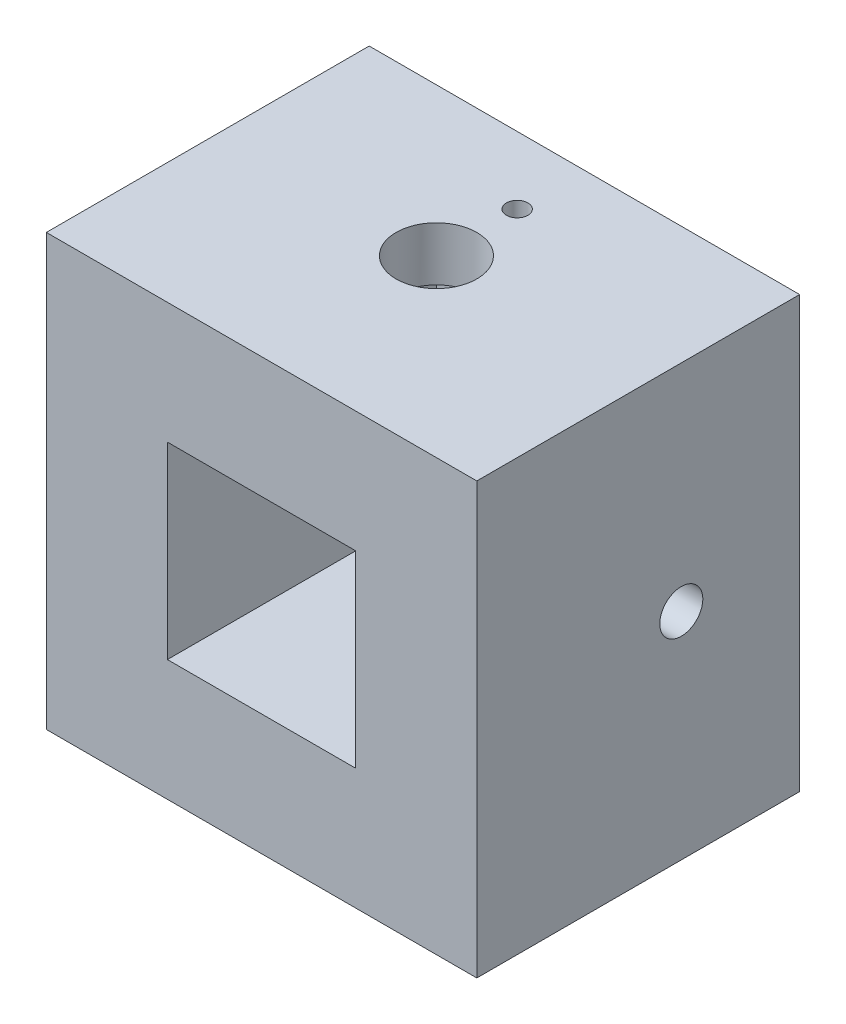
SolidWorks part; units mm, degrees
ref_plane "Front Plane" through (0, 0, 0) normal (0, 0, 1) x (1, 0, 0)
ref_plane "Top Plane" through (0, 0, 0) normal (0, 1, 0) x (1, 0, 0)
ref_plane "Right Plane" through (0, 0, 0) normal (1, 0, 0) x (0, 0, -1)
sketch "Sketch1" plane through (0, 0, 0) normal (0, 0, 1) x (1, 0, 0)
  line L1 (-51.5, -61.5) -> (-131.5, -61.5)
  line L2 (-51.5, -61.5) -> (-51.5, 18.5)
  line L3 (-51.5, 18.5) -> (-131.5, 18.5)
  line L4 (-131.5, -61.5) -> (-131.5, 18.5)
  line L5 (-51.5, -61.5) -> (-131.5, 18.5) construction
  line L6 (-51.5, 18.5) -> (-131.5, -61.5) construction
  point P0 (-91.5, -21.5)
  dimension "D1" = 80
  dimension "D2" = 80
extrude "Boss-Extrude1" add sketch "Sketch1" along normal blind 50 from offset 10
sketch "Sketch2" plane through (0, 0, 10) normal (0, 0, -1) x (-1, 0, 0)
  line L0 (91.5, 18.5) -> (91.5, -61.5) construction
  line L1 (74, -4) -> (109, -4)
  line L2 (74, -4) -> (74, -39)
  line L3 (74, -39) -> (109, -39)
  line L4 (109, -4) -> (109, -39)
  line L5 (74, -4) -> (109, -39) construction
  line L6 (74, -39) -> (109, -4) construction
  line L7 (51.5, 18.5) -> (131.5, 18.5) construction
  line L8 (131.5, -61.5) -> (51.5, -61.5) construction
  point P0 (91.5, -21.5)
  dimension "D1" = 35
  dimension "D2" = 35
extrude "Cut-Extrude1" cut sketch "Sketch2" against normal blind 45
sketch "Sketch3" plane through (0, 0, 10) normal (0, 0, -1) x (-1, 0, 0)
  line L8 (119, -49) -> (119, 6)
  line L9 (119, 6) -> (64, 6)
  line L10 (64, 6) -> (64, -49)
  line L11 (64, -49) -> (119, -49)
  line L12 (119, -49) -> (119, 6)
  line L13 (119, 6) -> (64, 6)
  line L14 (64, 6) -> (64, -49)
  line L15 (64, -49) -> (119, -49)
  dimension "D1" = 10
extrude "Cut-Extrude2" cut sketch "Sketch3" against normal blind 5
sketch "Sketch4" plane through (0, -61.5, 0) normal (0, -1, 0) x (-1, 0, 0)
  line L0 (91.5, -10) -> (91.5, -27.5) construction
  line L1 (131.5, -10) -> (51.5, -10) construction
  line L3 (84, -20) -> (99, -20)
  line L4 (84, -20) -> (84, -35)
  line L5 (84, -35) -> (99, -35)
  line L6 (99, -20) -> (99, -35)
  line L7 (84, -20) -> (99, -35) construction
  line L8 (84, -35) -> (99, -20) construction
  line L9 (131.5, -60) -> (51.5, -60) construction
  dimension "D1" = 15
  dimension "D2" = 15
  dimension "D3" = 25
extrude "Cut-Extrude3" cut sketch "Sketch4" against normal blind 156
sketch "Sketch5" plane through (0, -61.5, 0) normal (0, -1, 0) x (1, 0, 0)
  line L0 (-91.5, 20) -> (-91.5, 27.5) construction
  line L1 (-99, 20) -> (-84, 20) construction
  line L2 (-91.5, 27.5) -> (-99, 27.5) construction
  line L3 (-99, 35) -> (-99, 20) construction
  line L8 (-99, 20) -> (-84, 20)
  line L9 (-99, 35) -> (-99, 20)
  line L10 (-84, 35) -> (-99, 35)
  line L11 (-84, 20) -> (-84, 35)
  line L12 (-99, 20) -> (-84, 20)
  line L13 (-99, 35) -> (-99, 20)
  line L14 (-84, 35) -> (-99, 35)
  line L15 (-84, 20) -> (-84, 35)
  circle A0 centre (-91.5, 27.5) radius 7.5
  line M6 (-84, 20) -> (-99, 20)
  line M7 (-99, 20) -> (-99, 35)
  line M8 (-99, 35) -> (-84, 35)
  line M9 (-84, 35) -> (-84, 20)
  dimension "D1" = 0
extrude "Boss-Extrude2" add sketch "Sketch5" against normal blind 10 contours A0 L12 M7 | A0 L15 M6 | A0 L14 M9 | A0 L13 M8
sketch "Sketch6" plane through (0, 18.5, 0) normal (0, 1, 0) x (1, 0, 0)
  line L4 (-84, -20) -> (-99, -20)
  line L5 (-84, -35) -> (-84, -20)
  line L6 (-99, -35) -> (-84, -35)
  line L7 (-99, -20) -> (-99, -35)
  line L8 (-84, -20) -> (-99, -20)
  line L9 (-84, -35) -> (-84, -20)
  line L10 (-99, -35) -> (-84, -35)
  line L11 (-99, -20) -> (-99, -35)
  circle A1 centre (-91.5, -27.5) radius 7.5
  circle A2 centre (-91.5, -27.5) radius 7.5
  line M6 (-84, -35) -> (-99, -35)
  line M7 (-99, -35) -> (-99, -20)
  line M8 (-99, -20) -> (-84, -20)
  line M9 (-84, -20) -> (-84, -35)
  dimension "D1" = 0
  dimension "D2" = 0
extrude "Boss-Extrude3" add sketch "Sketch6" against normal blind 10 contours A2 L8 M9 | A2 L11 M8 | A2 L10 M7 | A2 L9 M6
sketch "Sketch9" plane through (-131.5, 0, 0) normal (-1, 0, 0) x (0, 0, 1)
  line L0 (10, -21.5) -> (22, -21.5) construction
  line L1 (10, 18.5) -> (10, -61.5) construction
  circle A0 centre (22, -21.5) radius 4
  dimension "D1" = 8
  dimension "D2" = 12
extrude "Cut-Extrude6" cut sketch "Sketch9" against normal blind 99
sketch "Sketch13" plane through (0, 0, 55) normal (0, 0, -1) x (-1, 0, 0)
  line L4 (109, -39) -> (109, -4)
  line L5 (109, -4) -> (74, -4)
  line L6 (74, -4) -> (74, -39)
  line L7 (74, -39) -> (109, -39)
  line L8 (109, -39) -> (109, -4)
  line L9 (109, -4) -> (74, -4)
  line L10 (74, -4) -> (74, -39)
  line L11 (74, -39) -> (109, -39)
  dimension "D1" = 0
extrude "Cut-Extrude7" cut sketch "Sketch13" against normal blind 200
ref_plane "Plane1" through (-91.5, 0, 0) normal (-1, 0, 0) x (0, 0, 1)
sketch "Sketch14" plane through (0, -49, 0) normal (0, 1, 0) x (1, 0, 0)
  line L0 (-91.5, -10) -> (-91.5, -15) construction
  line L1 (-51.5, -10) -> (-131.5, -10) construction
  line L2 (-64, -15) -> (-119, -15) construction
  circle A0 centre (-91.5, -12.5) radius 2
  dimension "D1" = 4
extrude "Cut-Extrude8" cut sketch "Sketch14" against normal blind 43 and the other way through all
sketch "Sketch15" plane through (0, 0, 10) normal (0, 0, -1) x (-1, 0, 0)
  line L0 (64, -49) -> (119, -49) construction
  line L1 (119, -49) -> (119, 6) construction
  line L2 (64, 6) -> (64, -49) construction
  line L3 (119, 6) -> (64, 6) construction
  line L4 (131.5, -61.5) -> (131.5, 18.5)
  line L5 (131.5, 18.5) -> (51.5, 18.5)
  line L6 (51.5, 18.5) -> (51.5, -61.5)
  line L7 (51.5, -61.5) -> (131.5, -61.5)
  line L8 (131.5, -61.5) -> (131.5, 18.5)
  line L9 (131.5, 18.5) -> (51.5, 18.5)
  line L10 (51.5, 18.5) -> (51.5, -61.5)
  line L11 (51.5, -61.5) -> (131.5, -61.5)
  line L12 (64, -49) -> (119, -49)
  line L13 (119, -49) -> (119, 6)
  line L14 (64, 6) -> (64, -49)
  line L15 (119, 6) -> (64, 6)
  dimension "D1" = 0
extrude "Boss-Extrude4" add sketch "Sketch15" along normal blind 10
